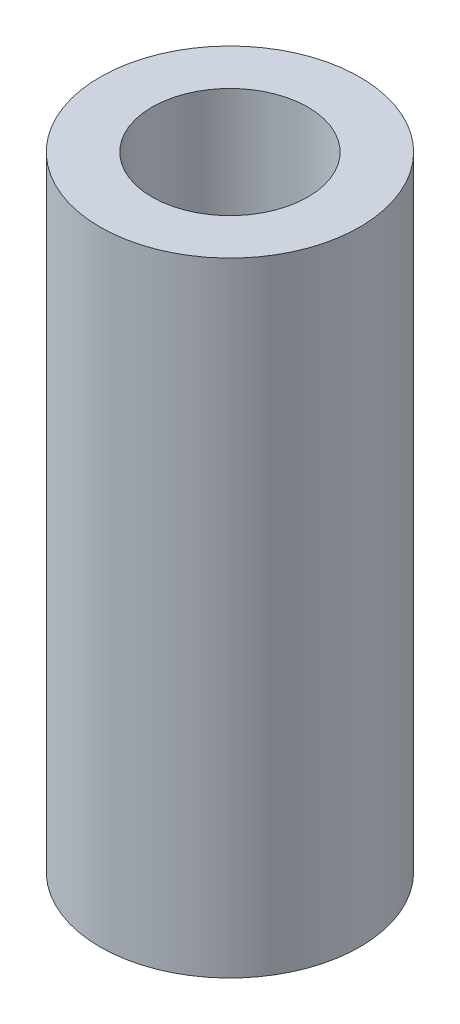
SolidWorks part; units mm, degrees
material "6061 合金"
ref_plane "前视基准面" through (0, 0, 0) normal (0, 0, 1) x (1, 0, 0)
ref_plane "上视基准面" through (0, 0, 0) normal (0, 1, 0) x (1, 0, 0)
ref_plane "右视基准面" through (0, 0, 0) normal (1, 0, 0) x (0, 0, -1)
other "Configuration Table"
sketch "草图1" plane through (0, 0, 0) normal (0, 1, 0) x (1, 0, 0)
  circle A0 centre (0, 0) radius 2.5
  circle A1 centre (0, 0) radius 1.5
  dimension "D1" = 3
  dimension "D2" = 5
extrude "凸台-拉伸1" add sketch "草图1" along normal blind 12
